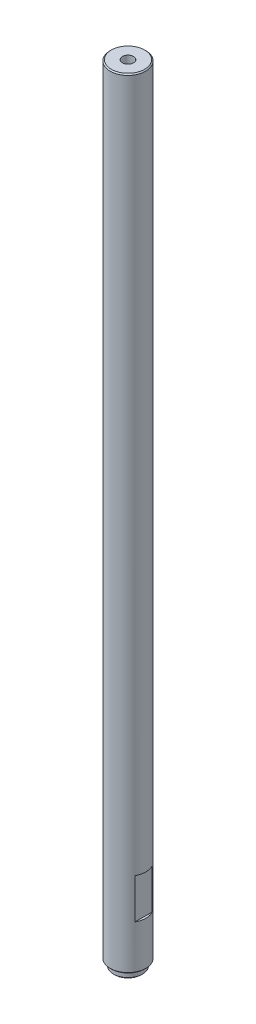
from build123d import *

# Parameters (mm, degrees)
SKETCH1_R             = 8
BOSS_EXTRUDE1_DEPTH   = 175
CUT_EXTRUDE1_START    = -20
SKETCH8_OUTSIDE_W     = 88.146
SKETCH8_OUTSIDE_H     = 88.146
SKETCH8_OUTSIDE_W_2   = 14
SKETCH8_OUTSIDE_H_2   = 30.19056833
CUT_EXTRUDE1_DEPTH    = 18
SKETCH9_R             = 6.5
BOSS_EXTRUDE2_DEPTH   = 3
M6_TAPPED_HOLE2_D     = 5
M6_TAPPED_HOLE2_DEPTH = 17
M6_TAPPED_HOLE2_TIP   = 1.502151548
CHAMFER1_SIZE         = 0.5
CHAMFER2_SIZE         = 0.5


with BuildPart() as part:
    # Sketch1 → Boss-Extrude1 (new, symmetric)
    with BuildSketch(Plane(origin=(0, 0, 0), x_dir=(1, 0, 0), z_dir=(0, 1, 0))):
        with Locations(Location((0, 0, 0), (0, 0, 270))):
            Circle(SKETCH1_R)
    extrude(amount=BOSS_EXTRUDE1_DEPTH, both=True)

    # Sketch7 → M6 Tapped Hole1 (revolve, cut)
    with BuildSketch(Plane(origin=(0, 175, 0), x_dir=(0, 0, 1), z_dir=(1, 0, 0))):
        Polygon((0, 0), (0, 16.502151548), (2.5, 15), (2.5, 0), align=None)
    m6_tapped_hole1 = revolve(axis=Axis((0, 181.35, 0), (0, -1, 0)), mode=Mode.SUBTRACT)

    # Mirror1: M6 Tapped Hole1 across plane
    add(m6_tapped_hole1.mirror(Plane.ZX), mode=Mode.SUBTRACT)

    # Sketch8 outside → Cut-Extrude1 (cut)
    with BuildSketch(Plane.XZ.offset(175).offset(CUT_EXTRUDE1_START)):
        Rectangle(SKETCH8_OUTSIDE_W, SKETCH8_OUTSIDE_H)
        Rectangle(SKETCH8_OUTSIDE_W_2, SKETCH8_OUTSIDE_H_2, mode=Mode.SUBTRACT)
    extrude(amount=-CUT_EXTRUDE1_DEPTH, mode=Mode.SUBTRACT)

    # Sketch9 → Boss-Extrude2 (add)
    with BuildSketch(Plane.XZ.offset(175)):
        with Locations(Location((0, 0, 0), (0, 0, 270))):
            Circle(SKETCH9_R)
    extrude(amount=BOSS_EXTRUDE2_DEPTH)

    # M6 Tapped Hole2
    with Locations(Plane(origin=(0, -178, 0), x_dir=(-1, 0, 0), z_dir=(0, -1, 0))):
        with Locations((0, 0)):
            Hole(M6_TAPPED_HOLE2_D / 2, depth=M6_TAPPED_HOLE2_DEPTH)
            with Locations((0, 0, -(M6_TAPPED_HOLE2_DEPTH + M6_TAPPED_HOLE2_TIP / 2))):  # 118° drill point
                Cone(0, M6_TAPPED_HOLE2_D / 2, M6_TAPPED_HOLE2_TIP, mode=Mode.SUBTRACT)

    # Chamfer1
    chamfer1_edges = [part.edges().sort_by_distance(p)[0] for p in [
        (0, -175, -8),
        (0, -178, 6.5),
    ]]
    chamfer(chamfer1_edges, length=CHAMFER1_SIZE)

    # Chamfer2
    chamfer2_edges = [part.edges().sort_by_distance(p)[0] for p in [
        (0, 175, -8),
    ]]
    chamfer(chamfer2_edges, length=CHAMFER2_SIZE)


solid = part.part
